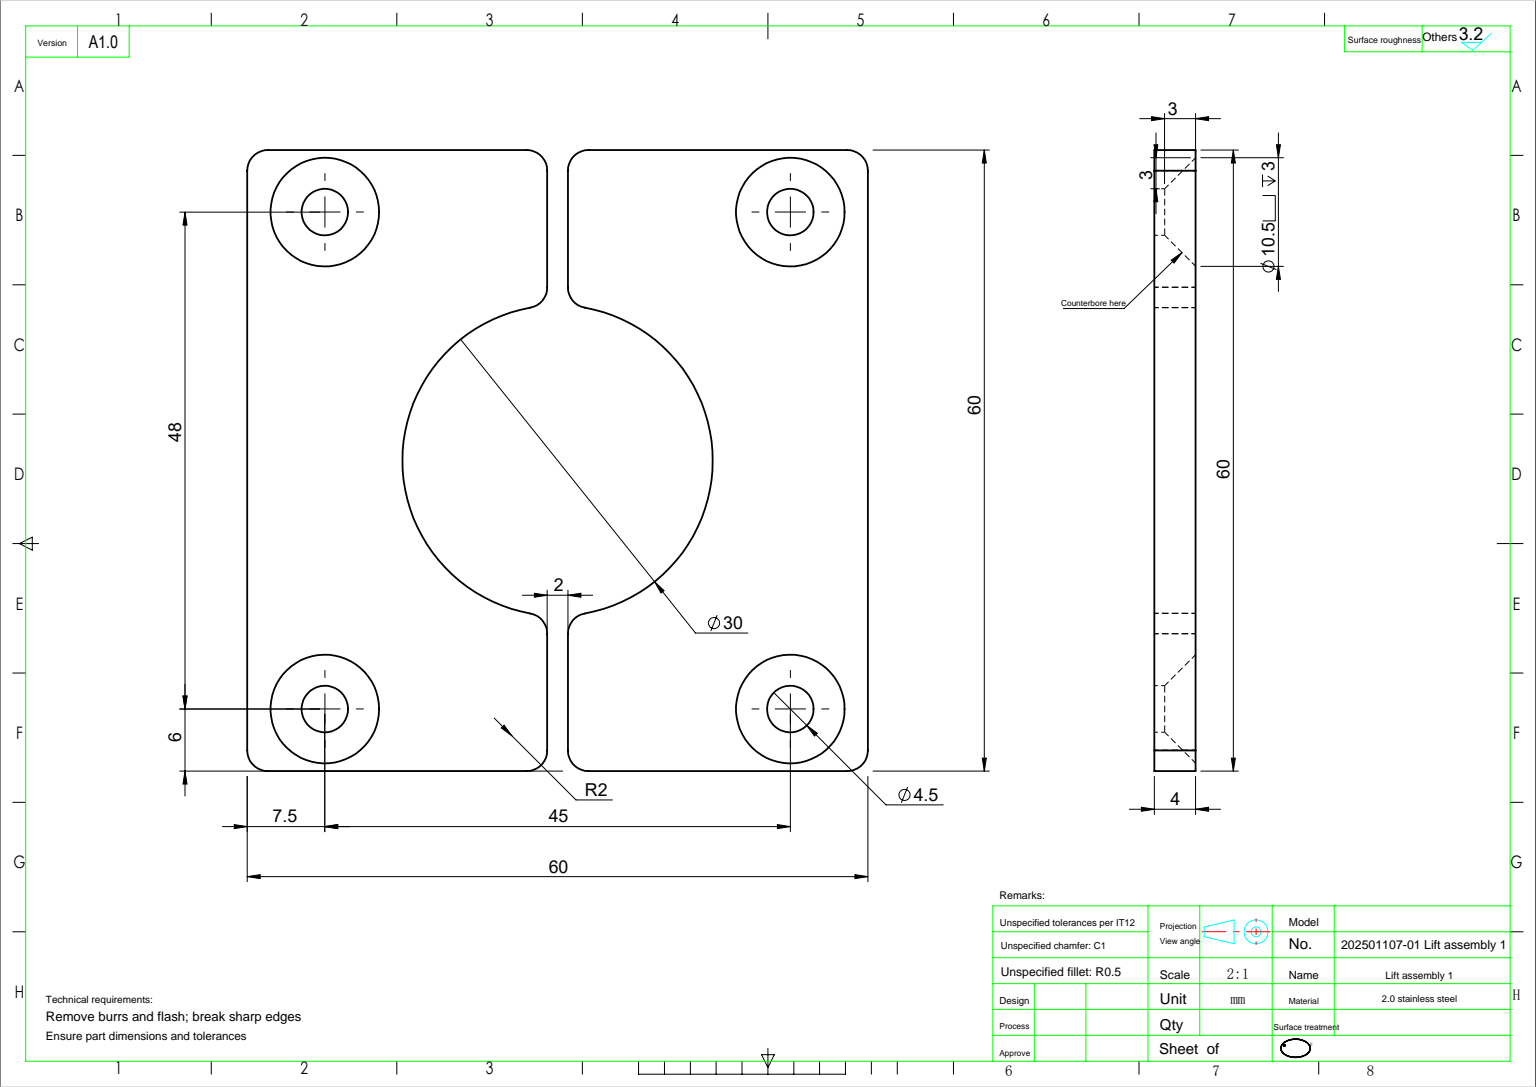
from build123d import *

# Parameters (mm, degrees)
SKETCH_1_W          = 60
SKETCH_1_H          = 60
SKETCH_1_R          = 15
EXTRUDE_1_DEPTH     = 4
SKETCH_2_W          = 2
SKETCH_2_H          = 73.723220536
CUT_EXTRUDE_1_DEPTH = 20
SKETCH_3_R          = 2.25
CUT_EXTRUDE_2_DEPTH = 10
CHAMFER_1_SIZE      = 3
CHAMFER_2_SIZE      = 3
FILLET_1_R          = 2
FILLET_2_R          = 2


with BuildPart() as part:
    # 草图1 → 凸台-拉伸1 (new body)
    with BuildSketch(Plane.XY):
        Rectangle(SKETCH_1_W, SKETCH_1_H)
        Circle(SKETCH_1_R, mode=Mode.SUBTRACT)
    extrude(amount=EXTRUDE_1_DEPTH)

    # 草图2 → 切除-拉伸1 (cut)
    with BuildSketch(Plane.XY.offset(4)):
        Rectangle(SKETCH_2_W, SKETCH_2_H)
    extrude(amount=-CUT_EXTRUDE_1_DEPTH, mode=Mode.SUBTRACT)


with BuildPart() as cut_extrude_1_piece_1:
    # of the separate pieces the step leaves, piece 1, a body of its own (cut_extrude_1_pieces)
    add(part.part.solids().sort_by_distance((-30, 30, 0))[0])


with BuildPart() as cut_extrude_1_piece_2:
    # of the separate pieces the step leaves, piece 2, a body of its own (cut_extrude_1_pieces)
    add(part.part.solids().sort_by_distance((1, 30, 0))[0])


with BuildPart() as cut_extrude_2_tool:
    # 草图3 → 切除-拉伸2 (new body)
    with BuildSketch(Plane.XY.offset(4)):
        with Locations((-22.5, 24)):
            Circle(SKETCH_3_R)
        with Locations((22.5, 24)):
            Circle(SKETCH_3_R)
        with Locations((-22.5, -24)):
            Circle(SKETCH_3_R)
        with Locations((22.5, -24)):
            Circle(SKETCH_3_R)
    extrude(amount=-CUT_EXTRUDE_2_DEPTH)


with BuildPart() as cut_extrude_1_piece_1_1:
    add(cut_extrude_1_piece_1.part)

    # 切除-拉伸2: cut by cut_extrude_2_tool
    add(cut_extrude_2_tool.part, mode=Mode.SUBTRACT)

    # 倒角1
    chamfer_1_edges = [cut_extrude_1_piece_1_1.edges().sort_by_distance(p)[0] for p in [
        (-24.75, 24, 4),
        (-24.75, -24, 4),
    ]]
    chamfer(chamfer_1_edges, length=CHAMFER_1_SIZE)

    # 圆角2
    fillet_2_edges = [cut_extrude_1_piece_1_1.edges().sort_by_distance(p)[0] for p in [
        (-1, -14.966629547, 2),
        (-1, 14.966629547, 2),
        (-1, 30, 2),
        (-1, -30, 2),
        (-30, -30, 2),
        (-30, 30, 2),
    ]]
    fillet(fillet_2_edges, radius=FILLET_2_R)


with BuildPart() as cut_extrude_1_piece_2_1:
    add(cut_extrude_1_piece_2.part)

    # 切除-拉伸2: cut by cut_extrude_2_tool
    add(cut_extrude_2_tool.part, mode=Mode.SUBTRACT)

    # 倒角2
    chamfer_2_edges = [cut_extrude_1_piece_2_1.edges().sort_by_distance(p)[0] for p in [
        (20.25, 24, 4),
        (20.25, -24, 4),
    ]]
    chamfer(chamfer_2_edges, length=CHAMFER_2_SIZE)

    # 圆角1
    fillet_1_edges = [cut_extrude_1_piece_2_1.edges().sort_by_distance(p)[0] for p in [
        (1, 30, 2),
        (30, 30, 2),
        (1, -30, 2),
        (30, -30, 2),
        (1, 14.966629547, 2),
        (1, -14.966629547, 2),
    ]]
    fillet(fillet_1_edges, radius=FILLET_1_R)


solid = Compound([cut_extrude_1_piece_1_1.part, cut_extrude_1_piece_2_1.part])
